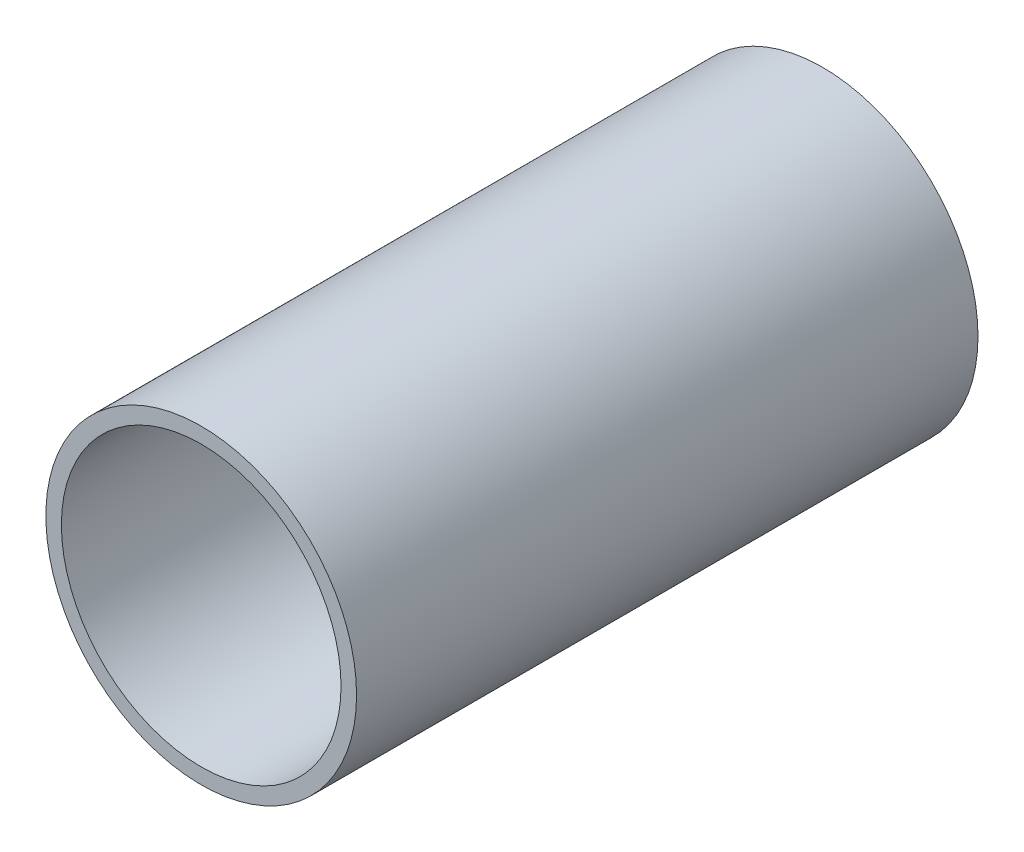
from build123d import *

# Parameters (mm, degrees)
SKETCH_1_R      = 20
SKETCH_1_R_2    = 18
EXTRUDE_1_DEPTH = 40


with BuildPart() as part:
    # 草图1 → 凸台-拉伸1 (new, symmetric)
    with BuildSketch(Plane.XY):
        Circle(SKETCH_1_R)
        Circle(SKETCH_1_R_2, mode=Mode.SUBTRACT)
    extrude(amount=EXTRUDE_1_DEPTH, both=True)


solid = part.part
